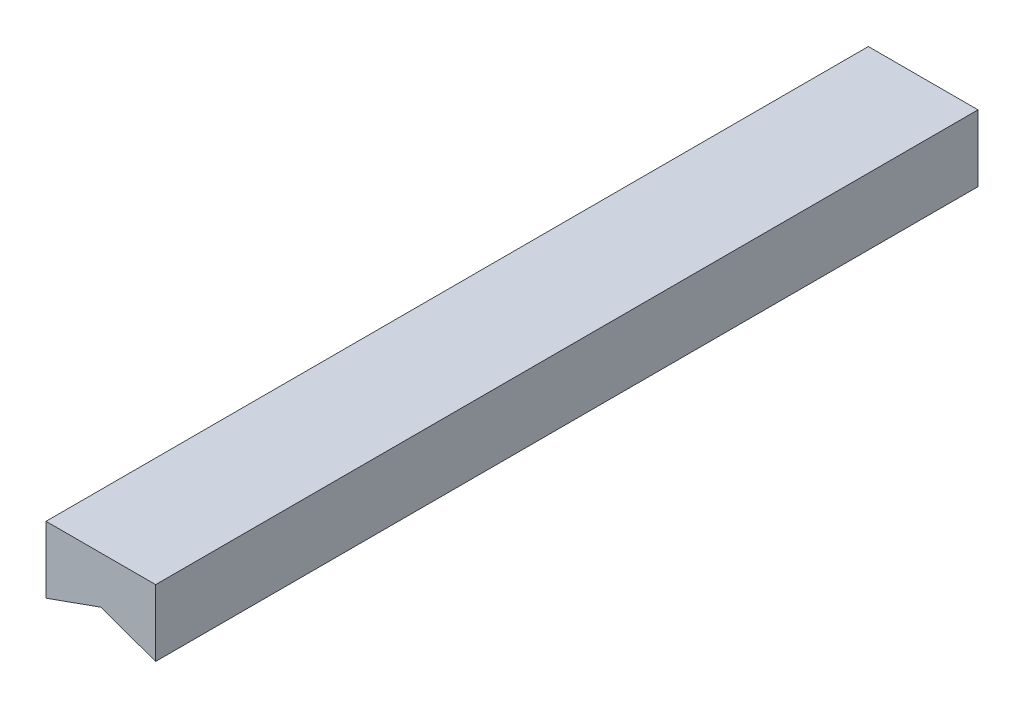
SolidWorks part; units mm, degrees
ref_plane "前视基准面" through (0, 0, 0) normal (0, 0, 1) x (1, 0, 0)
ref_plane "上视基准面" through (0, 0, 0) normal (0, 1, 0) x (1, 0, 0)
ref_plane "右视基准面" through (0, 0, 0) normal (1, 0, 0) x (0, 0, -1)
sketch "草图1" plane through (0, 0, 0) normal (0, 0, 1) x (1, 0, 0)
  line L0 (0, 0) -> (-14, -5)
  line L1 (-14, -5) -> (-14, 12)
  line L2 (-14, 12) -> (14, 12)
  line L3 (14, 12) -> (14, -5)
  line L4 (14, -5) -> (0, 0)
  line L5 (0, 0) -> (0, 12) construction
  dimension "D1" = 28
  dimension "D2" = 12
  dimension "D3" = 5
extrude "凸台-拉伸1" add sketch "草图1" along normal mid plane 210
